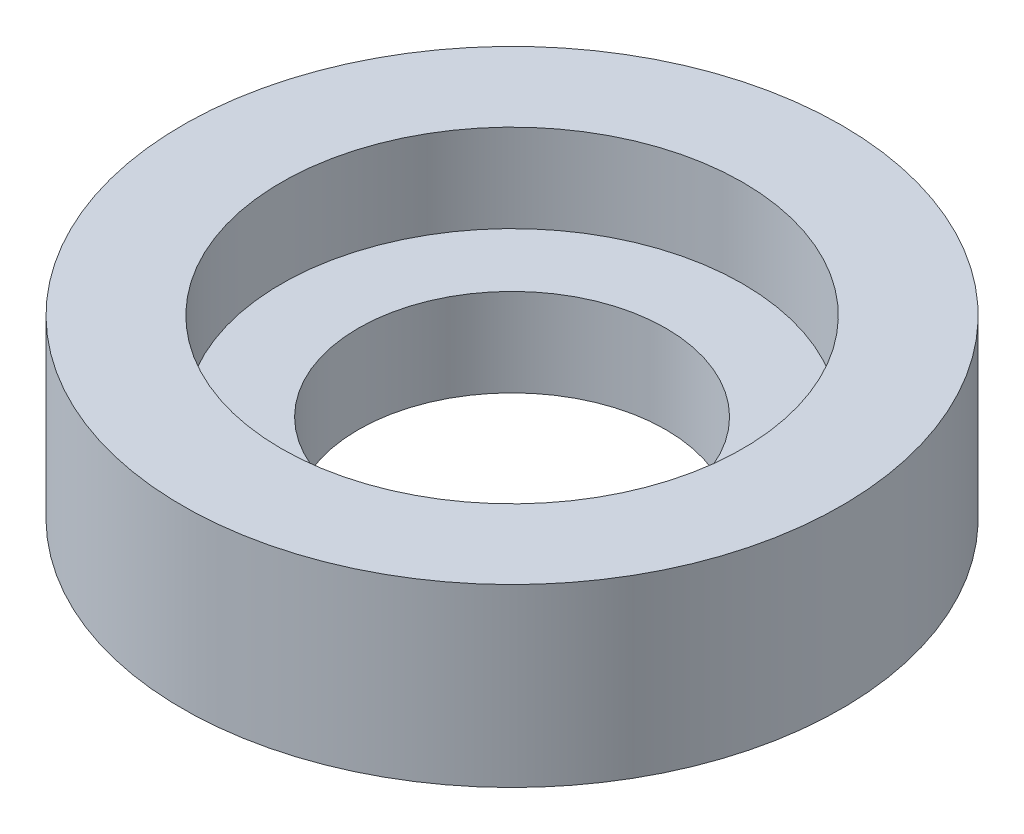
from build123d import *


with BuildPart() as part:
    # Sketch1 → Revolve1 (revolve)
    with BuildSketch(Plane.XY, mode=Mode.PRIVATE) as revolve1_sk:
        Polygon((-3.5, 0), (-7.5, 0), (-7.5, 4), (-5.25, 4), (-5.25, 2), (-3.5, 2), align=None)
    revolve(revolve1_sk.sketch.rotate(Axis((0, 0, 0), (0, 1, 0)), 270), axis=Axis((0, 0, 0), (0, 1, 0)))


solid = part.part
